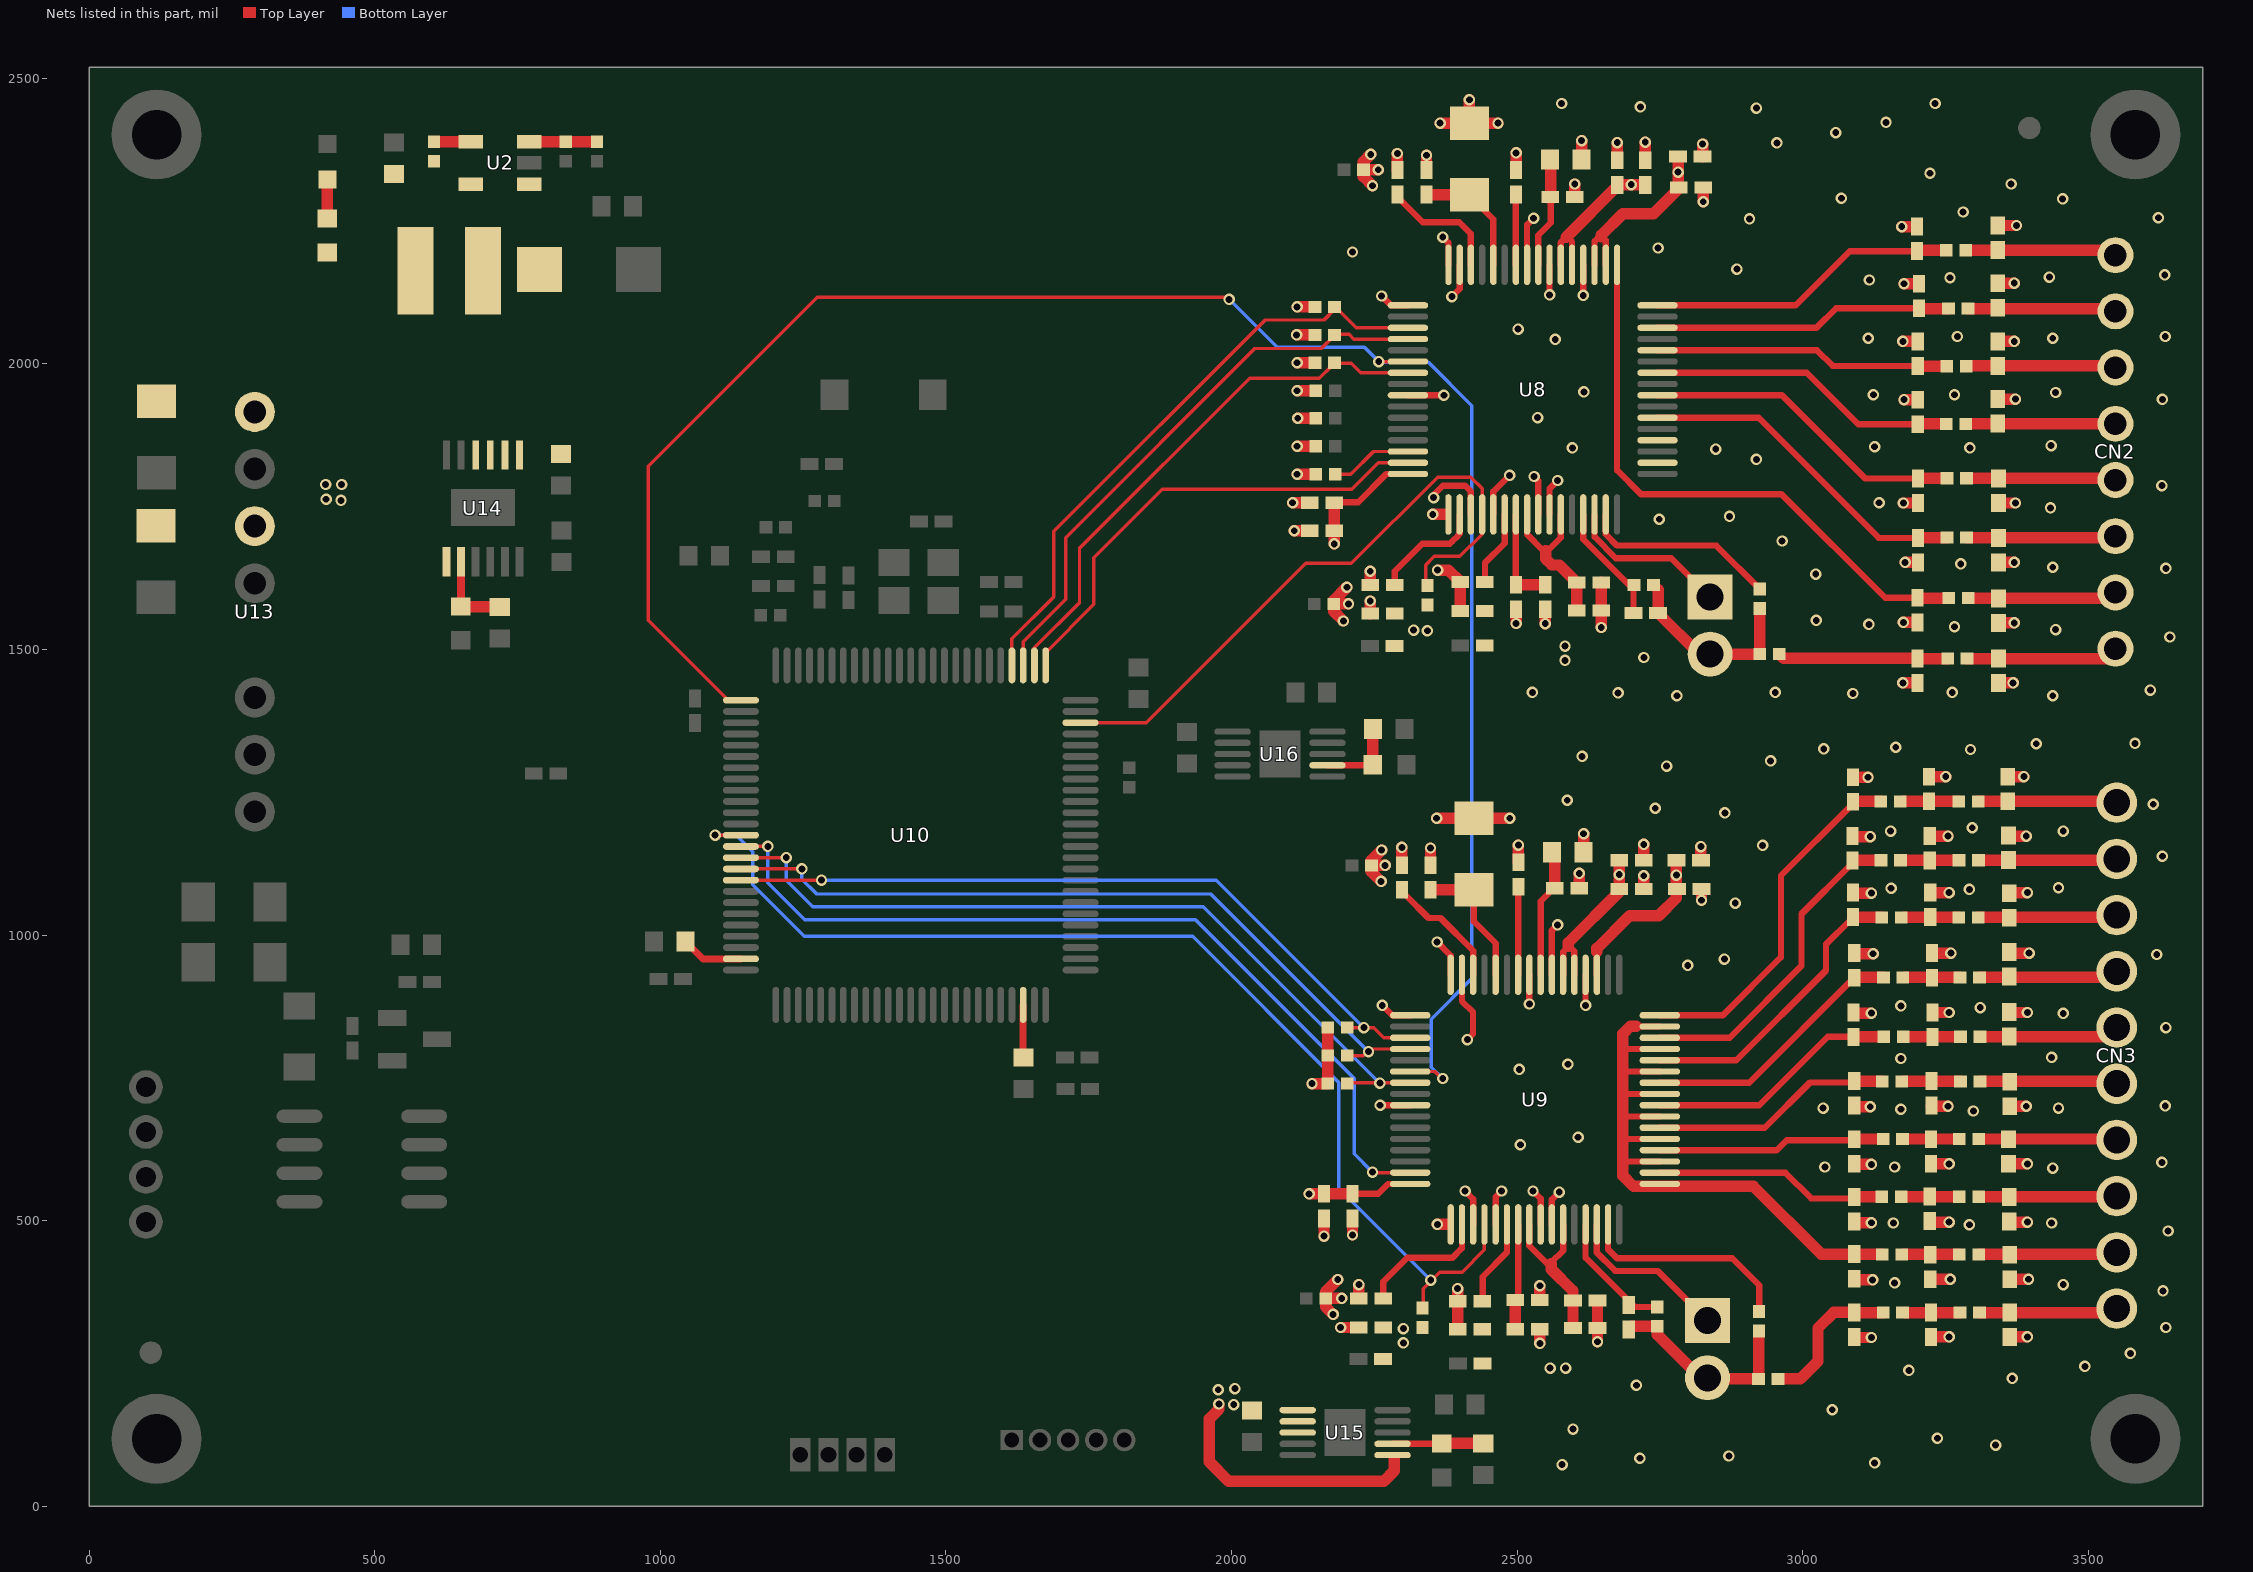
[diagram p0: the nets of this part, all layers, seen from the top]
# Altium PCB MISC86293.PcbDoc (part 3 of 4)
Units mil, origin at the board's own origin, x right, y up, seen from the top; angles counter-clockwise.
Board outline 3700.79 x 2519.68 mil, 4 copper layers (Top Layer, GND, POWER, Bottom Layer); 211 components, 128 nets, 717 pads, 581 vias.

## Via types
v1: diameter 20, hole 12, Top Layer to Bottom Layer, 581 vias

## Nets (pads, with @x,y where several pads share a name; then routed paths per layer and width w, separated by ;. In a path a pad name is that pad's centre, name@x,y a point inside that pad or via, vN(x,y) a via of type N, cw(c..) or ccw(c..) an arc to the next point about the centre after c; other vN are vias at no path point) (continued)
ADS_START: U8.38 U9.38 U10.26 | length 3457.3
  Top Layer w6: U10.26@1141.24,1411.22 1118.78,1411.22 979,1551 979,1821 1275,2117 1844,2117 ; 1848,2117 1844,2117 ; v1@1992,2117 1844,2117 ; v1(2257.79,2004.21) U8.38@2308.98,2004.21 ; U9.38@2312.98,761.21 2355.79,761.21 v1@2367,750
  Bottom Layer w6: v1(1996,2113) 2080,2029 2233,2029 2249,2013 v1(2257.79,2004.21) 2259,2003 2345,2003 2421,1927 2421,924 2350,853 2350,769 v1(2370,749)
DVCC_5V: C6.2 C109.1 C112.2 C118.2 L1.2 R1.1 R3.2 U2.5 U13.6 U14.1 U14.2 U14.3 U14.4 U14.7 U15.1 U15.2 U15.3 U15.6 | length 473.6
  Top Layer w20: v1(1978,179) 1978,170 1961,153 1961,78 1995,44 2267,44 2285,62 2285,82
  other v1: 2004,178 1977,204 2006,206 441,1761 415,1763 414,1789 442,1789
EEG_A1: C50.2 R25.2 U8.8 | length 566.8
  Top Layer w11: U8.8@2745.98,1945.16 2963.84,1945.16 3109.54,1799.46 C50.2@3201.96,1799.46
  Top Layer w20: C50.2@3202.5,1800 R25.2@3252.92,1800
EEG_A2: U8.4
EEG_AVDD: C30.2 C31.2 C32.1 C33.1 C34.2 C35.2 C36.2 C37.2 L3.2 U8.18 U8.19 U8.21 U8.22 U8.54 U8.56 U8.59 | length 1010.5
  Top Layer w11: C33.1@2444,1624 2444,1652 2478.27,1686.27 U8.54@2478.27,1736.5 ; U8.56@2517.64,1736.5 2517.64,1701.36 2544,1675 ; 2554,1673 2576.69,1695.69 U8.59@2576.69,1736.5 ; U8.22@2576.69,2173.5 2576.69,2212.69 2585,2221 ; 2591,2219 2596.38,2213.62 U8.21@2596.38,2173.5 ; U8.19@2635.75,2173.5 2635.75,2214.75 2645,2224 ; 2650,2222 2655.43,2216.57 U8.18@2655.43,2173.5
  Top Layer w20: 2550,1673 2550,1659 2561,1648 2574.02,1648 C36.2@2604.54,1617.48 C37.2@2604.54,1572.54 ; 2586,2222 2675.48,2311.48 C30.2@2675.48,2313.54 ; 2647,2223 2647,2225 2685,2263 2739,2263 2782.02,2306.02 C35.2@2782.02,2363 ; C30.2@2676.54,2313.54 C31.2@2724.48,2313.54
  other v1: 2584,1481 2584,1506 2700,2314 2782,2336
EEG_AVSS: C24.2 C25.1 C26.1 C27.1 C28.1 C29.2 C30.1 C31.1 C32.2 C33.2 C34.1 C35.1 C36.1 C37.1 C42.1 C43.1 C44.1 C45.1 C46.1 C47.1 C48.1 C49.1 C50.1 C51.1 D2.1 D3.1 D4.1 D5.1 D6.1 D7.1 D8.1 D9.1 R6.1 U8.20 U8.23 U8.25 U8.32 U8.53 U8.57 U8.58 | length 1605
  Top Layer w11: v1(2370,2222) 2379.84,2212.16 U8.32@2379.84,2173.5 ; U8.53@2458.58,1736.5 2458.58,1776.58 v1(2487,1805) ; U8.25@2517.64,2173.5 2517.64,2243.64 v1(2529,2255) ; v1(2530,1803) 2537.32,1795.68 U8.57@2537.32,1736.5 ; U8.58@2557.01,1736.5 2557.01,1782.01 v1(2571,1796) ; v1(2557.01,2121.01) U8.23@2557.01,2173.5 ; v1(2616.06,2119.94) U8.20@2616.06,2173.5
  Top Layer w20: v1(2244,2367) 2231.04,2354.04 R6.1@2231.04,2340 ; v1(2247,2312) 2231.04,2327.96 R6.1@2231.04,2340 ; v1(2257,2340) R6.1@2231.04,2340 ; C24.2@2290.48,2339.46 v1(2290.48,2368.52) ; C25.1@2341.48,2339.46 v1(2341.48,2365.48) ; v1(2361,1639) 2380.06,1639 C33.2@2400.54,1618.52 ; v1(2365.3,2421.7) C26.1@2416.48,2421.7 ; C32.2@2400.54,1567.52 C33.2@2400.54,1616.46 ; v1(2416.48,2462.52) C26.1@2416.48,2421.7 ; v1(2466.7,2421.7) C26.1@2416.48,2421.7 ; v1(2498.48,1545.52) C27.1@2498.48,1570.54 ; C29.2@2498.48,2339.46 v1(2498.48,2369.52) ; v1(2549.48,1545.48) C28.1@2549.48,1570.54 ; C43.1@2600.94,2292 v1(2600.94,2315.06) ; C42.1@2613.04,2358 v1(2613.04,2391.04) ; v1(2647.46,1538.54) C36.1@2647.46,1617.48 ; C30.1@2675.48,2356.46 v1(2675.48,2387.48) ; C31.1@2724.48,2356.46 v1(2724.48,2388.52) ; C35.1@2824.94,2363 v1(2824.94,2385.06) ; v1(2825.94,2284.06) C34.1@2825.94,2309 ; v1(3173.46,2240.46) C47.1@3200.48,2240.46 ; v1(3175.54,1441.54) C44.1@3200.96,1441.54 ; v1(3175.54,2039.46) C48.1@3201.48,2039.46 ; v1(3176.46,1547.54) C45.1@3200.96,1547.54 ; v1(3176.46,1756.54) C50.1@3201.96,1756.54 ; v1(3177.46,1937.46) C49.1@3201.48,1937.46 ; v1(3177.46,2140.46) C46.1@3203.48,2140.46 ; v1(3179.46,1652.54) C51.1@3201.96,1652.54 ; D7.1@3341.48,1938.46 v1(3372.54,1938.46) ; D6.1@3341.48,2039.46 v1(3370.46,2039.46) ; D4.1@3341.48,2141.46 v1(3370.46,2141.46) ; D5.1@3342,2242.46 v1(3374.54,2242.46) ; D2.1@3342.96,1441.54 v1(3368.54,1441.54) ; D3.1@3342.96,1546.54 v1(3370.46,1546.54) ; D9.1@3342.96,1652.54 v1(3370.46,1652.54) ; D8.1@3342.96,1756.54 v1(3372.46,1756.54)
  other v1: 2780,1419 3438,1419 3088,1423 2677,1424 2527,1425 2952,1425 3262,1425 3609,1429 2722,1486 3643,1522 3443,1535 3266,1540 3116,1544 3024,1551 3023,1632 3636,1642 3438,1644 3277,1650 2964,1690 2749,1728 2872,1733 3434,1748 3134,1757 3629,1787 2919,1833 2848,1851 2597,1853 3293,1853 3126,1855 3435,1857 2536,1906 3630,1938 3124,1946 3266,1946 3443,1950 2617,1951 2567,2043 3115,2045 3438,2045 3271,2048 3635,2048 2502,2061 3117,2147 3258,2151 3432,2152 3634,2156 2885,2166 2747,2203 2907,2254 3623,2256 3281,2266 3455.26,2288.91 3068,2290 3365,2315 3223,2334 2955,2387 3058,2405 3146,2423 2919,2448 2716,2450 2578,2456 3232,2456
EEG_BAISIN: H1.1 U8.62 | length 285.1
  Top Layer w11: U8.62@2635.75,1736.5 2635.75,1697.29 2673.04,1660 2770,1660 H1.1@2838,1592
EEG_BAISINV: C23.2 R8.1 U8.61 | length 208.9
  Top Layer w11: U8.61@2616.06,1736.5 2616.06,1692.94 2704.02,1604.98 C23.2@2704.02,1564
EEG_BAISIOUT: R9.1 U8.63 | length 344
  Top Layer w11: U8.63@2655.43,1736.5 2655.43,1701.65 2675.08,1682 2849.04,1682 R9.1@2925,1606.04
EEG_BIAS: C44.2 R10.2 R19.2 | length 297.5
  Top Layer w20: R10.2@2959.04,1492 2966.58,1484.46 C44.2@3200.96,1484.46 ; C44.2@3201.42,1484 R19.2@3253.92,1484
EEG_CLKSEL: R15.1 U8.52 U10.98 | length 1102.8
  Top Layer w6: U10.98@1735.72,1371.85 1850.85,1371.85 2130,1651 2210,1651 2361,1802 2419,1802 2439,1782 U8.52@2439,1758 ; R15.1@2343,1616 2340,1619 2340,1648 2355,1663 2400,1663 2438.9,1701.9 U8.52@2438.9,1736.5
EEG_CZ: C49.2 R24.2 U8.10 | length 542.3
  Top Layer w11: U8.10@2745.98,1984.53 3007.47,1984.53 3097.46,1894.54 C49.2@3201.48,1894.54
  Top Layer w20: C49.2@3201.94,1895 R24.2@3251.44,1895
EEG_DGND: C38.2 C39.2 C40.1 C41.1 R11.2 R12.2 R13.2 R14.2 R58.1 U8.31 U8.33 U8.41 U8.49 U8.51 | length 652.8
  Top Layer w11: v1(2263,2119) 2279.36,2102.64 U8.33@2308.98,2102.64 ; U8.41@2308.98,1945.16 v1(2371.84,1945.16) ; v1(2354,1766) 2354,1771 2370,1787 2409,1787 2419.21,1776.79 U8.51@2419.21,1736.5 ; v1(2386,2118) 2399.53,2131.53 U8.31@2399.53,2173.5
  Top Layer w20: v1(2107,1757) C39.2@2137.02,1757 ; v1(2110,1708) C38.2@2137.02,1708 ; v1(2115,1807) R11.2@2147.44,1807 ; v1(2115,1856) R12.2@2147.44,1856 ; v1(2115,1953) R14.2@2147.44,1953 ; v1(2116,1905) R13.2@2147.44,1905 ; v1(2196,1550) 2179.04,1566.96 R58.1@2179.04,1580 ; v1(2202,1609) 2179.04,1586.04 R58.1@2179.04,1580 ; v1(2205,1580) R58.1@2179.04,1580 ; C41.1@2243.02,1563 v1(2243.02,1584.98) ; C40.1@2243.02,1613 v1(2243.02,1636.98) ; v1(2352.5,1736.5) 2374,1736.5
  other v1: 2212,2196
EEG_DRDY: U8.47 U10.1 | length 803
  Top Layer w6: U10.1@1674.7,1494.7 1759,1579 1759,1661 1879,1781 2211,1781 2257,1827 U8.47@2292,1827
EEG_DVDD: C38.1 C39.1 C40.2 C41.2 L4.2 R15.2 R16.2 R17.2 R18.2 U8.48 U8.50 | length 503.5
  Top Layer w11: C39.1@2185,1758 2222,1758 2271.36,1807.36 U8.48@2308.98,1807.36 ; C40.2@2286,1618 2286,1637 2334,1685 2382,1685 2386.57,1689.57 2386.89,1689.57 2396.85,1699.53 2396.85,1699.85 2399.53,1702.53 U8.50@2399.53,1736.5
  Top Layer w20: v1(2114,2051) R17.2@2146.44,2051 ; v1(2115,2002) R18.2@2146.44,2002 ; v1(2115,2100) R16.2@2146.44,2100 ; v1(2179.94,1685.06) C38.1@2179.94,1708 C39.1@2179.94,1754.94
  other v1: 2343,1533 2319,1534
EEG_EOGN: C47.2 R22.2 U8.16 | length 543.3
  Top Layer w11: U8.16@2745.98,2102.64 2987.64,2102.64 3082.54,2197.54 C47.2@3200.48,2197.54
  Top Layer w20: C47.2@3201.94,2199 R22.2@3251.44,2199
EEG_EOGP: C46.2 R21.2 U8.14 | length 523.1
  Top Layer w11: U8.14@2745.98,2063.27 3024.27,2063.27 3058.54,2097.54 C46.2@3203.48,2097.54
  Top Layer w20: C46.2@3204.02,2097 R21.2@3255.44,2097
EEG_FZ: C48.2 R23.2 U8.12 | length 517.3
  Top Layer w11: U8.12@2745.98,2023.9 3025.1,2023.9 3052.46,1996.54 C48.2@3201.48,1996.54
  Top Layer w20: C48.2@3202.02,1996 R23.2@3252.44,1996
EEG_O1: U8.2
EEG_PWDN: R16.1 U8.35 U10.4 | length 1054.8
  Top Layer w6: U10.4@1615.65,1472.24 1615.65,1518.65 1689,1592 1689,1707 2059,2077 2162,2077 R16.1@2180,2095 ; R16.1@2185,2097 2218.73,2063.27 U8.35@2308.98,2063.27
EEG_PZ: C51.2 R26.2 U8.6 | length 593.5
  Top Layer w11: U8.6@2745.98,1905.79 2923.21,1905.79 3133.54,1695.46 C51.2@3201.96,1695.46
  Top Layer w20: C51.2@3202.5,1696 R26.2@3252.92,1696
EEG_REF: C45.2 R20.2 U8.17 | length 1032.5
  Top Layer w11: U8.17@2675.12,2173.5 2675.12,1813.88 2717,1772 2963,1772 3144.54,1590.46 C45.2@3200.96,1590.46
  Top Layer w20: C45.2@3201.42,1590 R20.2@3255.92,1590
EEG_RESET: R17.1 U8.36 U10.3 | length 997
  Top Layer w6: U10.3@1635.33,1472.24 1635.33,1513.33 1710,1588 1710,1696 2041,2027 2157,2027 R17.1@2178,2048 ; R17.1@2186,2052 2206,2052 2214.42,2043.58 U8.36@2308.98,2043.58 ; R17.1@2187,2045 R17.1@2188.42,2043.58
EEG_SPI_CS: R18.1 U8.39 U10.2 | length 942.8
  Top Layer w6: U10.2@1655.02,1472.24 1655.02,1503.02 1734,1582 1734,1677 2032,1975 2154,1975 R18.1@2176,1997 ; R18.1@2185,2001 2210,2001 2226.47,1984.53 2258,1984.53 U8.39@2308.98,1984.53
EEG_VCAP1: C25.2 C26.2 U8.28 | length 184
  Top Layer w11: C26.2@2431,2281 2458.58,2253.42 U8.28@2458.58,2173.5
  Top Layer w20: C25.2@2341.48,2296.54 C26.2@2406.54,2296.54
EEG_VCAP2: C24.1 U8.30 | length 200.6
  Top Layer w11: C24.1@2297,2286 2335,2248 2399,2248 2419.21,2227.79 U8.30@2419.21,2173.5
EEG_VCAP3: C27.2 C28.2 U8.55 | length 164.5
  Top Layer w11: C27.2@2497.95,1621.05 U8.55@2497.95,1736.5
  Top Layer w20: C27.2@2500.46,1613.46 C28.2@2549.48,1613.46
EEG_VCAP4: C29.1 U8.26 | length 118.5
  Top Layer w11: U8.26@2497.95,2173.5 C29.1@2497.95,2291.95
EEG_VREFP: C42.2 C43.2 U8.24 | length 187.5
  Top Layer w11: U8.24@2537.32,2173.5 2537.32,2225.32 2559,2247 C43.2@2559,2288
  Top Layer w20: C43.2@2559,2288 C42.2@2559,2352
ELEC_EEG_A1: CN2.5 D8.2 R25.1 | length 257.6
  Top Layer w20: R25.1@3287,1800 CN2.5@3544.57,1800
ELEC_EEG_BIAS: CN2.8 D2.2 R19.1 | length 242.3
  Top Layer w20: R19.1@3288,1484 CN2.8@3530.27,1484
ELEC_EEG_CZ: CN2.4 D7.2 R24.1 | length 262.1
  Top Layer w20: R24.1@3285.52,1895 CN2.4@3547.57,1895
ELEC_EEG_EOGN: CN2.1 D5.2 R22.1 | length 265.8
  Top Layer w20: R22.1@3285.52,2199 3539.27,2199 CN2.1@3547.78,2190.49
ELEC_EEG_EOGP: CN2.2 D4.2 R21.1 | length 253.3
  Top Layer w20: R21.1@3289.52,2097 CN2.2@3542.84,2097
ELEC_EEG_FZ: CN2.3 D6.2 R23.1 | length 257.8
  Top Layer w20: R23.1@3287.06,1996.54 D6.2@3341.48,1996.54 CN2.3@3544.88,1996.54
ELEC_EEG_PZ: CN2.6 D9.2 R26.1 | length 258.4
  Top Layer w20: R26.1@3287,1696 CN2.6@3545.42,1696
ELEC_EEG_REF: CN2.7 D3.2 R20.1 | length 247.8
  Top Layer w20: R20.1@3290,1590 CN2.7@3537.84,1590
ELEC_EMG_C1: CN3.10 D10.2 R34.1 | length 215.5
  Top Layer w20: R34.1@3307.52,1234 CN3.10@3523,1234
ELEC_EMG_C2: CN3.9 D11.2 R36.1 | length 223.5
  Top Layer w20: R36.1@3309,1131 CN3.9@3532.48,1131
ELEC_EMG_C3: CN3.7 D12.2 R38.1 | length 231.5
  Top Layer w20: R38.1@3309.52,926 CN3.7@3541,926
ELEC_EMG_C4: CN3.8 D13.2 R40.1 | length 220.5
  Top Layer w20: R40.1@3307.52,1031 CN3.8@3528,1031
ELEC_EMG_RA: CN3.2 D18.2 R50.1 | length 234.5
  Top Layer w20: R50.1@3308.52,441 CN3.2@3543,441
ELEC_EMG_RL: CN3.1 D19.2 R52.1 | length 233.5
  Top Layer w20: R52.1@3309.52,339 CN3.1@3543,339
ELEC_EMG_V1: CN3.6 D14.2 R42.1 | length 221.5
  Top Layer w20: R42.1@3310.52,822 CN3.6@3532,822
ELEC_EMG_V2: CN3.5 D15.2 R44.1 | length 219.5
  Top Layer w20: R44.1@3310.52,744 CN3.5@3530,744
ELEC_EMG_V3: CN3.4 D16.2 R46.1 | length 215.5
  Top Layer w20: R46.1@3308.52,643 CN3.4@3524,643
ELEC_EMG_V4: CN3.3 D17.2 R48.1 | length 226.5
  Top Layer w20: R48.1@3308.52,542 CN3.3@3535,542
EMG_AVDD: C59.2 C60.2 C61.1 C62.1 C63.2 C64.2 C65.2 C66.2 L2.2 U9.19 U9.21 U9.22 U9.54 U9.56 U9.59 | length 1016.3
  Top Layer w11: C62.1@2440,365 2440,402 2482.27,444.27 U9.54@2482.27,493.5 ; U9.56@2521.64,493.5 2521.64,456.36 2554,424 ; 2560,427 2580.69,447.69 U9.59@2580.69,493.5 ; U9.22@2580.69,930.5 2580.69,970.69 2590,980 ; 2590,982 2600.38,971.62 U9.21@2600.38,930.5 ; U9.19@2639.75,930.5 2639.75,969.75
  Top Layer w20: 2560,425 2560,415 2598.02,376.98 C66.2@2598.02,360 C65.2@2598.02,312 ; 2590,980 2590,987 2679.02,1076.02 C60.2@2679.02,1081 C59.2@2679.02,1131 ; 2639.79,971.21 2639.79,976.79 2697,1034 2748,1034 2779.02,1065.02 C64.2@2779.02,1131
  other v1: 2558,242 2585,242 2779,1105 2679,1106
EMG_AVSS: C53.2 C54.1 C55.1 C56.1 C57.1 C58.2 C59.1 C60.1 C61.2 C62.2 C63.1 C64.1 C65.1 C66.1 C71.1 C72.1 C73.1 C74.1 C75.1 C76.1 C77.1 C78.1 C79.1 C80.1 C81.1 C82.1 C83.1 C84.1 C85.1 C86.1 C87.1 C88.1 C89.1 C90.1 C91.1 C92.1 D10.1 D11.1 D12.1 D13.1 D14.1 D15.1 D16.1 D17.1 D18.1 D19.1 R7.1 U9.20 U9.23 U9.25 U9.32 U9.53 U9.57 U9.58 | length 1943.3
  Top Layer w11: v1(2360,988) 2383.84,964.16 U9.32@2383.84,930.5 ; U9.53@2462.58,493.5 2462.58,541.58 v1(2473,552) ; v1(2521.64,879.36) U9.25@2521.64,930.5 ; v1(2528,552) 2541.32,538.68 U9.57@2541.32,493.5 ; U9.58@2561.01,493.5 2561.01,537.01 v1(2574,550) ; U9.23@2561.01,930.5 2561.01,1008.01 v1(2571,1018) ; v1(2620.06,876.94) U9.20@2620.06,930.5
  Top Layer w20: v1(2262,1094) 2245.04,1110.96 R7.1@2245.04,1122 ; v1(2263,1149) 2245.04,1131.04 R7.1@2245.04,1122 ; v1(2269,1122) R7.1@2245.04,1122 ; C53.2@2298.48,1122.46 v1(2298.48,1153.48) ; C54.1@2348.48,1122.46 v1(2348.48,1152.48) ; v1(2359.3,1204.7) C55.1@2424.48,1204.7 v1(2487.3,1204.7) ; C61.2@2396.02,310 v1(2396.02,380.98) ; C58.2@2502.48,1127.46 v1(2502.48,1157.48) ; v1(2539.94,285.06) C56.1@2539.94,310 ; C57.1@2539.94,361 v1(2539.94,386.06) ; C72.1@2608.94,1082 v1(2608.94,1107.94) ; C71.1@2616.56,1145 v1(2616.56,1177.56) ; v1(2640.94,287.94) C65.1@2640.94,312 ; C65.1@2640.94,314.94 C66.1@2640.94,360 ; C60.1@2721.94,1081 v1(2721.94,1103.94) ; C59.1@2721.94,1131 v1(2721.94,1158.94) ; C64.1@2821.94,1131 v1(2821.94,1154.94) ; v1(2822.94,1061.06) C63.1@2822.94,1081 ; C74.1@3088,1276.46 v1(3114.46,1276.46) ; C84.1@3092,699.46 v1(3118.46,699.46) ; C76.1@3092,1172.46 v1(3118.46,1172.46) ; C92.1@3094,295.46 v1(3120.46,295.46) ; C88.1@3094,496.46 v1(3120.46,496.46) ; C86.1@3094,598.46 v1(3120.46,598.46) ; C82.1@3094,863.46 v1(3120.46,863.46) ; C80.1@3094,1073.46 v1(3120.46,1073.46) ; C90.1@3096,396.46 v1(3122.46,396.46) ; C78.1@3097,967.46 v1(3123.46,967.46) ; C73.1@3221.48,1277.46 v1(3250.54,1277.46) ; C83.1@3225.48,700.46 v1(3254.54,700.46) ; C75.1@3225.48,1173.46 v1(3254.54,1173.46) ; C91.1@3227.48,296.46 v1(3256.54,296.46) ; C87.1@3227.48,497.46 v1(3256.54,497.46) ; C85.1@3227.48,599.46 v1(3256.54,599.46) ; C81.1@3227.48,864.46 v1(3256.54,864.46) ; C79.1@3227.48,1074.46 v1(3256.54,1074.46) ; C89.1@3229.48,397.46 v1(3258.54,397.46) ; C77.1@3230.48,968.46 v1(3259.54,968.46) ; D10.1@3359.48,1277.46 v1(3387.46,1277.46) ; D15.1@3363.48,700.46 v1(3391.46,700.46) ; D11.1@3363.48,1173.46 v1(3391.46,1173.46) ; D19.1@3365.48,296.46 v1(3393.46,296.46) ; D17.1@3365.48,497.46 v1(3393.46,497.46) ; D16.1@3365.48,599.46 v1(3393.46,599.46) ; D14.1@3365.48,864.46 v1(3393.46,864.46) ; D13.1@3365.48,1074.46 v1(3393.46,1074.46) ; D18.1@3367.48,397.46 v1(3395.46,397.46) ; D12.1@3368.48,968.46 v1(3396.46,968.46)
  other v1: 2579,73 3126,76 2715,84 2871,88 3338,107 3236,119 2598,135 3052,169 2709,212 3367,224 3186,238 3494.33,244.86 3574,267.75 3636,313 3631,377 3456.26,388 3161,391 3640,482 3292,493 3159,496 3436,496 3438,592 3039,594 3161,594 3629,602 2506,633 2607,646 3299,692 3172,695 3036,697 3448,697 3635,701 2504,765 2589,774 3172,784 3436,786 3636,838 3456.26,863 3311,873 3172,876 2799,947 2863,958 3620,966 2882,1056 3292,1080 3155,1082 3448,1083 3630,1138 2930,1157 3154,1182 3456.26,1182 3297,1188 2864,1214 2742,1222 3614,1229 2588,1236 2762,1296 2944,1305 2614,1313 3294,1325 3037,1326 3163,1329 3409,1335 3582,1335.57
EMG_C1: C74.2 R35.2 U9.16 | length 618.9
  Top Layer w11: U9.16@2749.98,859.64 2860.64,859.64 2962,961 2962,1104 C74.2@3085,1227 ; C74.2@3085,1232 C74.2@3087,1232
  Top Layer w20: C74.2@3091,1234 R35.2@3136.96,1234
EMG_C2: C76.2 R37.2 U9.14 | length 559.2
  Top Layer w11: U9.14@2749.98,820.27 2872.27,820.27 2998,946 2998,1037 C76.2@3084,1123
  Top Layer w20: C76.2@3091,1131 R37.2@3137.44,1131
EMG_C3: C78.2 R39.2 U9.10 | length 463.5
  Top Layer w11: U9.10@2749.98,741.53 2906.53,741.53 C78.2@3090,925
  Top Layer w20: C78.2@3094,926 R39.2@3141.44,926
EMG_C4: C80.2 R41.2 U9.12 | length 508.3
  Top Layer w11: U9.12@2749.98,780.9 2883.9,780.9 3041,938 3041,984 C80.2@3084,1027
  Top Layer w20: C80.2@3093,1031 R41.2@3138.44,1031
EMG_CLKSEL: R30.1 U9.52 U10.38 | length 1976.9
  Top Layer w6: v1(1096,1175) U10.38@1141.24,1175 ; R30.1@2336,348 2336,381 2365,410 2404,410 2442.9,448.9 U9.52@2442.9,493.5 ; v1(2349,396) v1@2350,396
  Bottom Layer w6: v1(1096,1175) 1133,1175 1162,1146 1162,1088 1252,998 1932,998 2188,742 2188,557 v1(2349,396)
EMG_DGND: C67.2 C68.2 C69.1 C70.1 R59.1 U9.31 U9.33 U9.41 U9.49 U9.51 | length 535.7
  Top Layer w11: v1(2260.16,702.16) U9.41@2312.98,702.16 ; v1(2264,877) 2281.36,859.64 U9.33@2312.98,859.64 ; U9.31@2403.53,930.5 2403.53,884.47 2423,865 2423,827 v1(2413,817) ; v1(2409,552) 2423.21,537.79 U9.51@2423.21,493.5
  Top Layer w20: v1(2162,473) C68.2@2162,504.06 ; v1(2178,336) 2165.04,348.96 R59.1@2165.04,364 ; v1(2186,397) 2165.04,376.04 R59.1@2165.04,364 ; v1(2191,313) C70.1@2223.02,313 ; v1(2193,364) R59.1@2165.04,364 ; v1(2212,475) C67.2@2212,504.06 ; C69.1@2223.02,364 v1(2223.02,387.98) ; v1(2360.5,493.5) 2378,493.5
EMG_DRDY: U9.47 U10.39 | length 1516.6
  Top Layer w6: U10.39@1141.24,1155.31 v1(1188.31,1155.31) ; v1@2252.95,584.05 U9.47@2312.98,584.05
  Bottom Layer w6: v1(1188.31,1155.31) 1188.31,1091.69 1253,1027 1937,1027 2215,749 2215,617 v1(2247,585)
EMG_DVDD: C67.1 C68.1 C69.2 C70.2 L5.2 R30.2 R31.2 R32.2 R33.2 U9.48 U9.50 | length 529.9
  Top Layer w11: C67.1@2218,547 2257,547 2274.36,564.36 U9.48@2312.98,564.36 ; C69.2@2266,369 2266,393 2308,435 2387,435 2403.53,451.53 U9.50@2403.53,493.5
  Top Layer w20: v1(2136.02,546.98) C68.1@2162,546.98 C67.1@2212,546.98 ; v1(2141,740) R33.2@2168.44,740 ; R33.2@2168.44,741.44 R32.2@2168.44,789 R31.2@2168.44,838
  other v1: 2301,286 2301,311
EMG_PWDN: R31.1 U9.35 U10.42 | length 1309.1
  Top Layer w6: U10.42@1141.24,1096.26 v1(1282.26,1096.26) ; R31.1@2209,838 2249,838 2266.73,820.27 U9.35@2312.98,820.27
  Bottom Layer w6: v1(1282.26,1096.26) 1973.74,1096.26 v1(2232,838)
EMG_RA: C90.2 R51.2 U9.1 U9.3 U9.5 U9.7 U9.9 U9.11 U9.13 U9.15 | length 1210
  Top Layer w11: 2685,603.73 U9.3@2749.98,603.73 ; 2685,643.1 U9.5@2749.98,643.1 ; 2685,682.47 U9.7@2749.98,682.47 ; 2685,721.84 U9.9@2749.98,721.84 ; 2685,761.21 U9.11@2749.98,761.21 ; 2685,800.58 U9.13@2749.98,800.58 ; 2714.05,839.95 U9.15@2749.98,839.95
  Top Layer w20: 2708.64,840.64 2698.64,840.64 2685,827 2685,800.58 2685,761.21 2685,721.84 2685,682.47 2685,643.1 2685,603.73 2685,579 2704,560 2914,560 3032.54,441.46 C90.2@3090.48,441.46 ; C90.2@3095,441 R51.2@3139.44,441
EMG_RESET: R32.1 U9.36 U10.41 | length 1353.5
  Top Layer w6: U10.41@1141.24,1115.94 v1(1247.94,1115.94) ; R32.1@2206,789 2231,789 2242.58,800.58 U9.36@2312.98,800.58
  Bottom Layer w6: v1(1247.94,1115.94) 1247.94,1098.06 1274,1072 1964,1072 v1(2240,796)
EMG_RL: C92.2 R29.2 R53.2 | length 260.7
  Top Layer w20: R29.2@2960,223 2996,223 3027,254 3027,312 3054.46,339.46 C92.2@3090.48,339.46 ; C92.2@3093,339 R53.2@3140.96,339
EMG_RLDIN: H2.1 U9.62 | length 249.5
  Top Layer w11: U9.62@2639.75,493.5 2639.75,444.25 2672,412 2746,412 H2.1@2803,355
EMG_RLDINV: C52.2 R27.1 U9.61 | length 218.1
  Top Layer w11: U9.61@2620.06,493.5 2620.06,434.94 2706,349 R27.1@2744,349
EMG_RLDOUT: R28.1 U9.63 | length 376.4
  Top Layer w11: U9.63@2659.43,493.5 2659.43,449.57 2675,434 2877,434 2924,387 R28.1@2924,345
EMG_SPI_CS: R33.1 U9.39 U10.40 | length 1411.7
  Top Layer w6: U10.40@1141.24,1135.63 v1(1220.63,1135.63) ; R33.1@2206.53,741.53 U9.39@2312.98,741.53
  Bottom Layer w6: v1(1220.63,1135.63) 1220.63,1096.37 1267,1050 1951,1050 v1(2260,741)
EMG_V1: C82.2 R43.2 U9.8 | length 433.6
  Top Layer w11: U9.8@2749.98,702.16 2924.16,702.16 3044,822 C82.2@3089,822
  Top Layer w20: C82.2@3097,822 R43.2@3141.96,822
EMG_V2: C84.2 R45.2 U9.6 | length 412.3
  Top Layer w11: U9.6@2749.98,662.79 2933.79,662.79 3013,742 C84.2@3090,742
  Top Layer w20: C84.2@3100,744 R45.2@3139.44,744
EMG_V3: C86.2 R47.2 U9.4 | length 386.3
  Top Layer w11: U9.4@2749.98,623.42 2954.42,623.42 2972,641 C86.2@3086,641
  Top Layer w20: C86.2@3098,643 R47.2@3140.96,643
EMG_V4: C88.2 R49.2 U9.2 | length 392.1
  Top Layer w11: U9.2@2749.98,584.05 2969.95,584.05 3015,539 C88.2@3083,539
  Top Layer w20: C88.2@3098,542 R49.2@3138.44,542
EMG_VCAP1: C54.2 C55.2 U9.28 | length 223.5
  Top Layer w11: C55.2@2424,1072 2424,1024 2462.58,985.42 U9.28@2462.58,930.5
  Top Layer w20: C54.2@2348.48,1079.54 C55.2@2414.54,1079.54
EMG_VCAP2: C53.1 U9.30 | length 200.8
  Top Layer w11: C53.1@2305,1070 2345,1030 2366,1030 2423.21,972.79 U9.30@2423.21,930.5
EMG_VCAP3: C56.2 C57.2 U9.55 | length 173.5
  Top Layer w11: C57.2@2501.95,364.95 U9.55@2501.95,493.5
  Top Layer w20: C56.2@2497.02,310 C57.2@2497.02,354.98
EMG_VCAP4: C58.1 U9.26 | length 144.5
  Top Layer w11: U9.26@2501.95,930.5 C58.1@2501.95,1075.05
EMG_VREFP: C71.2 C72.2 U9.24 | length 214.7
  Top Layer w11: U9.24@2541.32,930.5 2541.32,1059.32 C72.2@2564,1082
  Top Layer w20: C71.2@2564,1135 2566.02,1132.98 C72.2@2566.02,1082
NetC23_1: C23.1 H1.2 R8.2 R9.2 R10.1 | length 340
  Top Layer w20: R8.2@2739.04,1613 2746.94,1605.1 C23.1@2746.94,1564 2818.94,1492 R10.1@2924.96,1492 R9.2@2924.96,1571.92
NetC52_1: C52.1 H2.2 R27.2 R28.2 R29.1 | length 307.9
  Top Layer w20: C52.1@2700.96,314.96 R27.2@2745.48,314.96 2745.48,300.52 H2.2@2815,231 ; H2.2@2853,223 2917,223 2923.48,229.48 R28.2@2923.48,306.96
NetC73_2: C73.2 R34.2 R35.1 | length 97.4
  Top Layer w20: R35.1@3176,1234 R34.2@3273.44,1234
NetC75_2: C75.2 R36.2 R37.1 | length 96.5
  Top Layer w20: R37.1@3171.52,1131 R36.2@3268,1131
NetC77_2: C77.2 R38.2 R39.1 | length 95.4
  Top Layer w20: R39.1@3180,926 R38.2@3275.44,926
NetC79_2: C79.2 R40.2 R41.1 | length 94.4
  Top Layer w20: R41.1@3179,1031 R40.2@3273.44,1031
NetC81_2: C81.2 R42.2 R43.1 | length 91.4
  Top Layer w20: R43.1@3185,822 R42.2@3276.44,822
NetC83_2: C83.2 R44.2 R45.1 | length 99.4
  Top Layer w20: R45.1@3177,744 R44.2@3276.44,744
NetC85_2: C85.2 R46.2 R47.1 | length 92.4
  Top Layer w20: R47.1@3182,643 R46.2@3274.44,643
NetC87_2: C87.2 R48.2 R49.1 | length 96.4
  Top Layer w20: R49.1@3178,542 R48.2@3274.44,542
NetC89_2: C89.2 R50.2 R51.1 | length 97.4
  Top Layer w20: R51.1@3177,441 R50.2@3274.44,441
NetC91_2: C91.2 R52.2 R53.1 | length 95.4
  Top Layer w20: R53.1@3180,339 R52.2@3275.44,339
NetC96_2: C96.2 U10.73 | length 83.4
  Top Layer w12: C96.2@1635.33,794.33 U10.73@1635.33,877.76
NetC106_1: C106.1 U10.49 | length 98.6
  Top Layer w12: C106.1@1052,981 1074.54,958.46 U10.49@1141.24,958.46
NetC111_1: C111.1 U13.8
NetC114_2: C114.2 R60.2 U15.7 | length 147.8
  Top Layer w11: U15.7@2282.07,109.31 R60.2@2359.69,109.31
  Top Layer w20: R60.2@2371,110 2440.56,110 C114.2@2441,109.56
NetC116_2: C116.2 R61.1 U16.7 | length 131.2
  Top Layer w11: U16.7@2168.07,1297.31 R61.1@2239.69,1297.31
  Top Layer w20: R61.1@2247.44,1301.44 C116.2@2247.44,1361
NetC119_2: C119.2 R62.2 U14.8 | length 136.2
  Top Layer w14: R62.2@651.13,1582.87 U14.8@651.13,1653.5
  Top Layer w20: R62.2@653.44,1574.56 C119.2@719,1574.56
NetD1_2: D1.2 L1.1 U2.1
NetLED1_2: LED1.2 R1.2 | length 60.3
  Top Layer w20: R1.2@417,2254.66 LED1.2@417,2315
NetR3_1: R3.1 U2.4 | length 57.9
  Top Layer w20: R3.1@610.4,2389.4 U2.4@668.3,2389.4
NetR4_1: R4.1 R5.2 U2.3 | length 111.9
  Top Layer w20: U2.3@770.67,2389.4 R4.1@882.6,2389.4
NetR11_1: R11.1 U8.46 | length 139.4
  Top Layer w6: R11.1@2186,1807 2209,1807 2248.73,1846.73 U8.46@2308.98,1846.73